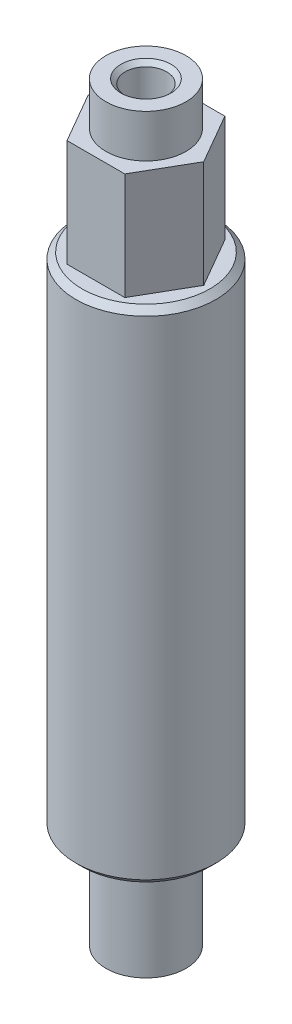
from build123d import *

# Parameters (mm, degrees)
BOSS_EXTRUDE1_DEPTH = 10.7
SKETCH3_W           = 4
SKETCH3_H           = 4.3


with BuildPart() as part:
    # Sketch1 → Revolve1 (revolve)
    with BuildSketch(Plane.XY, mode=Mode.PRIVATE) as revolve1_sk:
        Polygon((0, 110), (6.3865, 110), (7, 109.3865), (7, 60.6135), (6.3865, 60), (4, 60), (4, 50), (0, 50), align=None)
    revolve(revolve1_sk.sketch.rotate(Axis((0, 50, 0), (0, 1, 0)), 270), axis=Axis((0, 50, 0), (0, 1, 0)))

    # Sketch2 → Boss-Extrude1 (add)
    with BuildSketch(Plane(origin=(0, 110, 0), x_dir=(1, 0, 0), z_dir=(0, 1, 0))):
        Polygon((-5.773502692, 0), (-2.886751346, -5), (2.886751346, -5), (5.773502692, 0), (2.886751346, 5), (-2.886751346, 5), align=None)
    extrude(amount=BOSS_EXTRUDE1_DEPTH)

    # Sketch3 → Revolve2 (revolve)
    with BuildSketch(Plane.XY, mode=Mode.PRIVATE) as revolve2_sk:
        with Locations((2, 122.85)):
            Rectangle(SKETCH3_W, SKETCH3_H)
    revolve(revolve2_sk.sketch.rotate(Axis((0, 120.7, 0), (0, 1, 0)), 270), axis=Axis((0, 120.7, 0), (0, 1, 0)))

    # Sketch4 → Cut-Revolve1 (revolve, cut)
    with BuildSketch(Plane.XY, mode=Mode.PRIVATE) as cut_revolve1_sk:
        Polygon((0, 125), (2.5, 125), (2.067, 124.567), (2.067, 120), (2, 119.961317532), (2, 50), (0, 50), align=None)
    revolve(cut_revolve1_sk.sketch.rotate(Axis((0, 50, 0), (0, 1, 0)), 270), axis=Axis((0, 50, 0), (0, 1, 0)), mode=Mode.SUBTRACT)


solid = part.part
